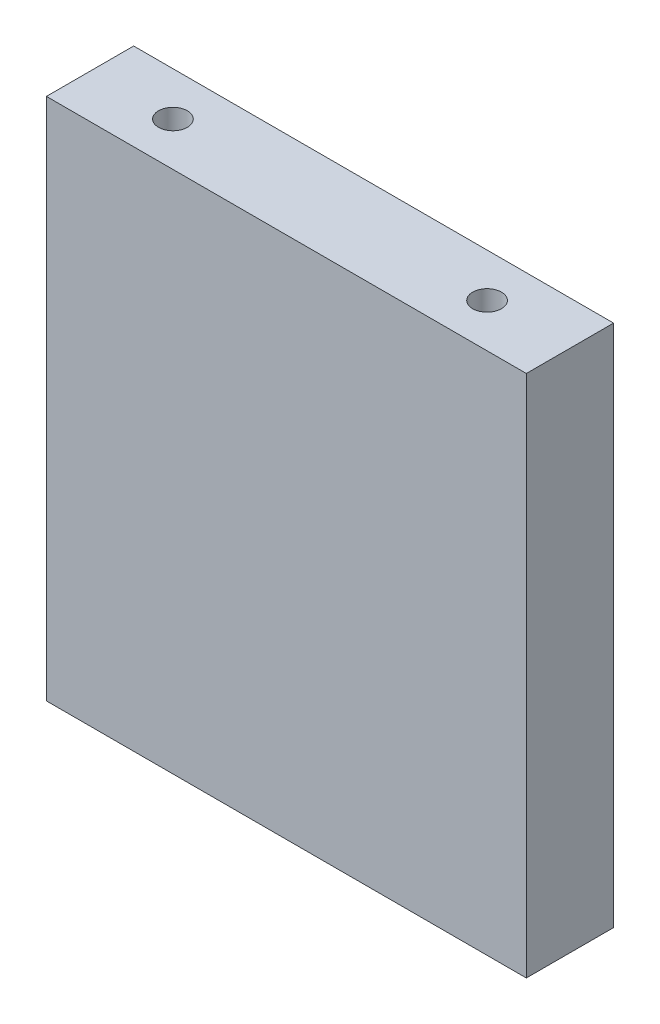
from build123d import *

# Parameters (mm, degrees)
SKETCH_1_W                  = 55
SKETCH_1_H                  = 60
EXTRUDE_1_DEPTH             = 5
HOLE_WIZARD_M4_1_AT_2_COUNT = 2
HOLE_WIZARD_M4_1_AT_2_PITCH = 36


with BuildPart() as part:
    # 草图1 → 凸台-拉伸1 (new, symmetric)
    with BuildSketch(Plane.XY):
        Rectangle(SKETCH_1_W, SKETCH_1_H)
    extrude(amount=EXTRUDE_1_DEPTH, both=True)

    # 草图4 → M4 螺纹孔1 (revolve, cut)
    with BuildSketch(Plane(origin=(18, -30, 0), x_dir=(0, 0, -1), z_dir=(1, 0, 0))):
        Polygon((0, 0), (0, 12.491420021), (1.65, 11.5), (1.65, 0), align=None)
    hole_wizard_m4_1 = revolve(axis=Axis((18, -36.35, 0), (0, 1, 0)), mode=Mode.SUBTRACT)

    # M4 螺纹孔1 at 2: M4 螺纹孔1 ×2
    with Locations(*[(-i * HOLE_WIZARD_M4_1_AT_2_PITCH, 0, 0) for i in range(1, HOLE_WIZARD_M4_1_AT_2_COUNT)]):
        add(hole_wizard_m4_1, mode=Mode.SUBTRACT)

    # 镜向1: M4 螺纹孔1 across plane
    add(hole_wizard_m4_1.mirror(Plane.ZX), mode=Mode.SUBTRACT)

    # 镜向1 copy 1 sketch → 镜向1 copy 1 (revolve, cut)
    with BuildSketch(Plane(origin=(-18, 30, 0), x_dir=(0, 0, -1), z_dir=(1, 0, 0))):
        Polygon((0, 0), (0, -12.491420021), (1.65, -11.5), (1.65, 0), align=None)
    revolve(axis=Axis((-18, 36.35, 0), (0, 1, 0)), mode=Mode.SUBTRACT)


solid = part.part
